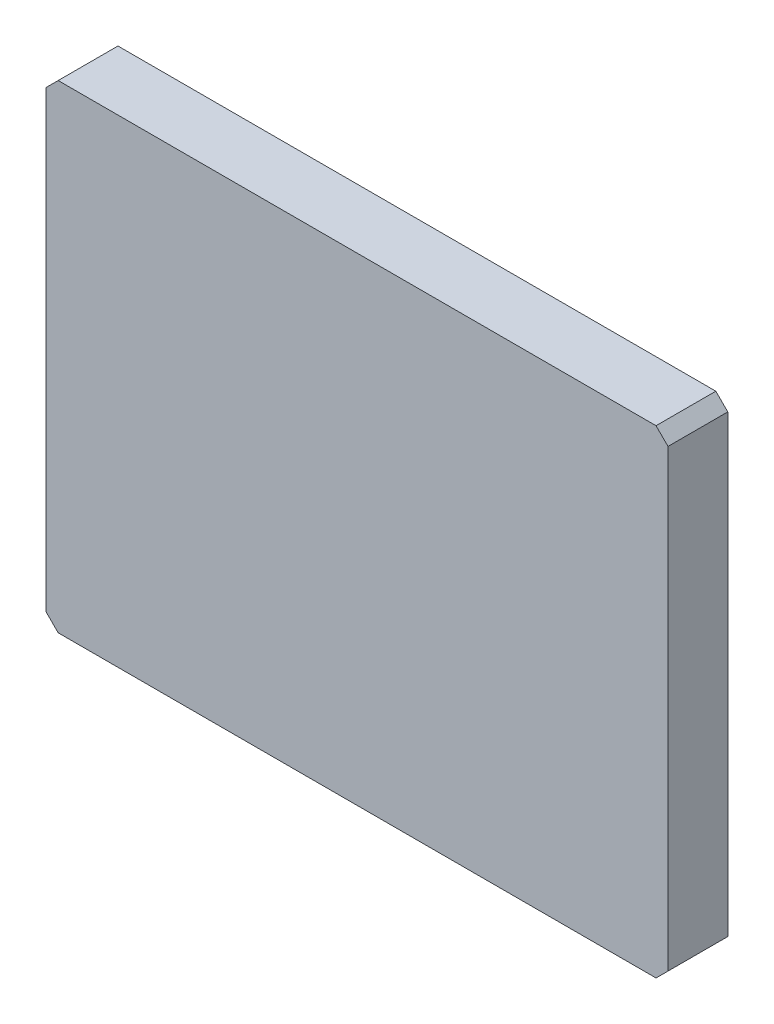
from build123d import *

# Parameters (mm, degrees)
SKETCH_1_W      = 260
SKETCH_1_H      = 200
EXTRUDE_1_DEPTH = 25
CHAMFER_1_SIZE  = 5


with BuildPart() as part:
    # 草图1 → 凸台-拉伸1 (new body)
    with BuildSketch(Plane.XY):
        Rectangle(SKETCH_1_W, SKETCH_1_H)
    extrude(amount=EXTRUDE_1_DEPTH)

    # 倒角1
    chamfer_1_edges = [part.edges().sort_by_distance(p)[0] for p in [
        (130, -100, 12.5),
        (-130, -100, 12.5),
        (-130, 100, 12.5),
        (130, 100, 12.5),
    ]]
    chamfer(chamfer_1_edges, length=CHAMFER_1_SIZE)


solid = part.part
